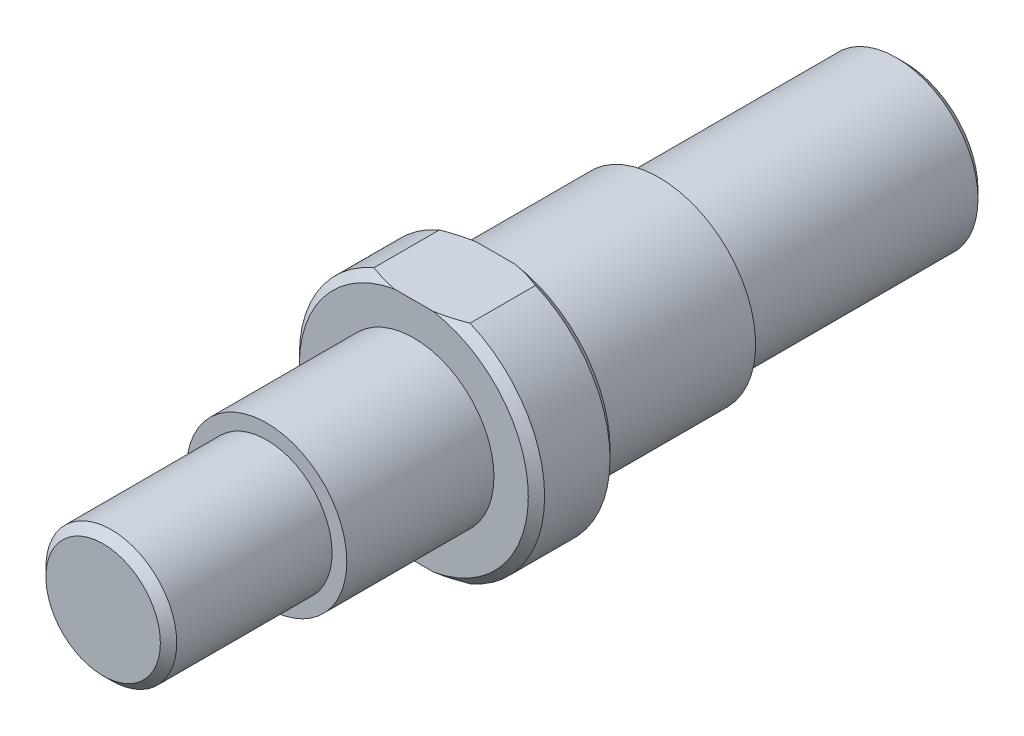
SolidWorks part; units mm, degrees
ref_plane "前视基准面" through (0, 0, 0) normal (0, 0, 1) x (1, 0, 0)
ref_plane "上视基准面" through (0, 0, 0) normal (0, 1, 0) x (1, 0, 0)
ref_plane "右视基准面" through (0, 0, 0) normal (1, 0, 0) x (0, 0, -1)
sketch "草图1" plane through (0, 0, 0) normal (0, 0, 1) x (1, 0, 0)
  circle A0 centre (0, 0) radius 7.5
  dimension "D1" = 15
extrude "凸台-拉伸1" add sketch "草图1" along normal mid plane 49
sketch "草图2" plane through (0, 0, 24.5) normal (0, 0, 1) x (1, 0, 0)
  circle A0 centre (0, 0) radius 4.9
  dimension "D1" = 9.8
extrude "切除-拉伸1" cut sketch "草图2" against normal blind 19 flip side to cut
sketch "草图3" plane through (0, 0, 24.5) normal (0, 0, 1) x (1, 0, 0)
  circle A0 centre (0, 0) radius 4
  dimension "D1" = 8
extrude "切除-拉伸2" cut sketch "草图3" against normal blind 10 flip side to cut
cosmetic thread "装饰螺纹线1" parameters "D2"=6.647
sketch "草图4" plane through (0, 0, -24.5) normal (0, 0, -1) x (-1, 0, 0)
  circle A0 centre (0, 0) radius 5.9
  dimension "D1" = 11.8
extrude "切除-拉伸3" cut sketch "草图4" against normal blind 25 flip side to cut
sketch "草图5" plane through (0, 0, -24.5) normal (0, 0, -1) x (-1, 0, 0)
  circle A0 centre (0, 0) radius 5
  dimension "D1" = 10
extrude "切除-拉伸4" cut sketch "草图5" against normal blind 15 flip side to cut
cosmetic thread "装饰螺纹线2" parameters "D2"=6.647
chamfer "倒角1" distance 0.5 angle 45 4 edges at (-7.5, 0, 0.5) (7.5, 0, 5.5) (4, 0, 24.5) (-5, 0, -24.5)
sketch "草图6" plane through (0, 0, 5.5) normal (0, 0, 1) x (1, 0, 0)
  line L0 (0, 0) -> (-11.1419, 0) construction
  line L1 (-7.5, 12.9) -> (7.5, 12.9)
  line L2 (-7.5, 12.9) -> (-7.5, 6.9)
  line L3 (-7.5, 6.9) -> (7.5, 6.9)
  line L4 (7.5, 12.9) -> (7.5, 6.9)
  line L5 (0, 0) -> (0, 13.0284) construction
  line L6 (7.5, -12.9) -> (7.5, -6.9)
  line L7 (-7.5, -6.9) -> (7.5, -6.9)
  line L8 (-7.5, -12.9) -> (-7.5, -6.9)
  line L9 (-7.5, -12.9) -> (7.5, -12.9)
  dimension "D1" = 15
  dimension "D2" = 6
  dimension "D3" = 13.8
extrude "切除-拉伸5" cut sketch "草图6" against normal blind 15
